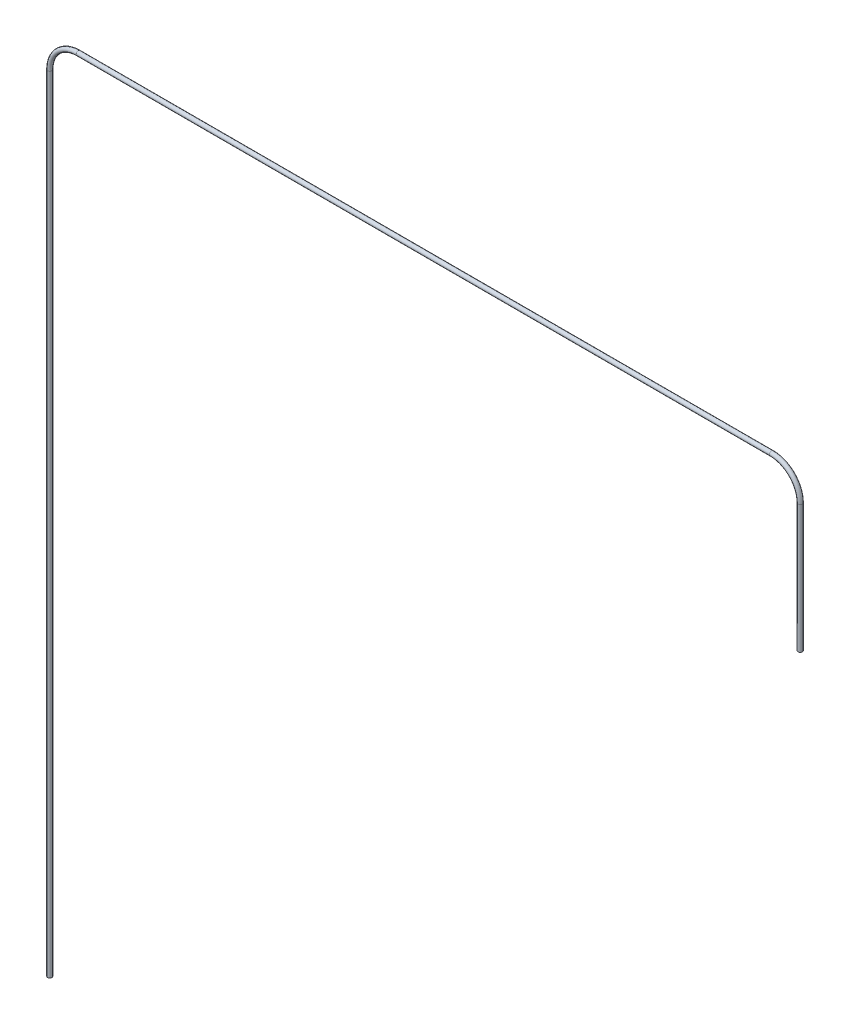
from build123d import *

# Parameters (mm, degrees)
SKETCH2_R = 3.25


with BuildPart() as part:
    # Sweep1: sweep along a path in Sketch1
    with BuildLine(Plane.XY) as sweep1_path:
        Line((0, 0), (0, 1153))
        ThreePointArc((0, 1153), (12.30151519, 1182.69848481), (42, 1195))
        Line((42, 1195), (1060, 1195))
        ThreePointArc((1060, 1195), (1089.69848481, 1182.69848481), (1102, 1153))
        Line((1102, 1153), (1102, 965))
    # Sketch2 → Sweep1 (sweep)
    with BuildSketch(Plane(origin=(0, 0, 0), x_dir=(1, 0, 0), z_dir=(0, 1, 0))):
        Circle(SKETCH2_R)
    sweep(path=sweep1_path.line)


solid = part.part
